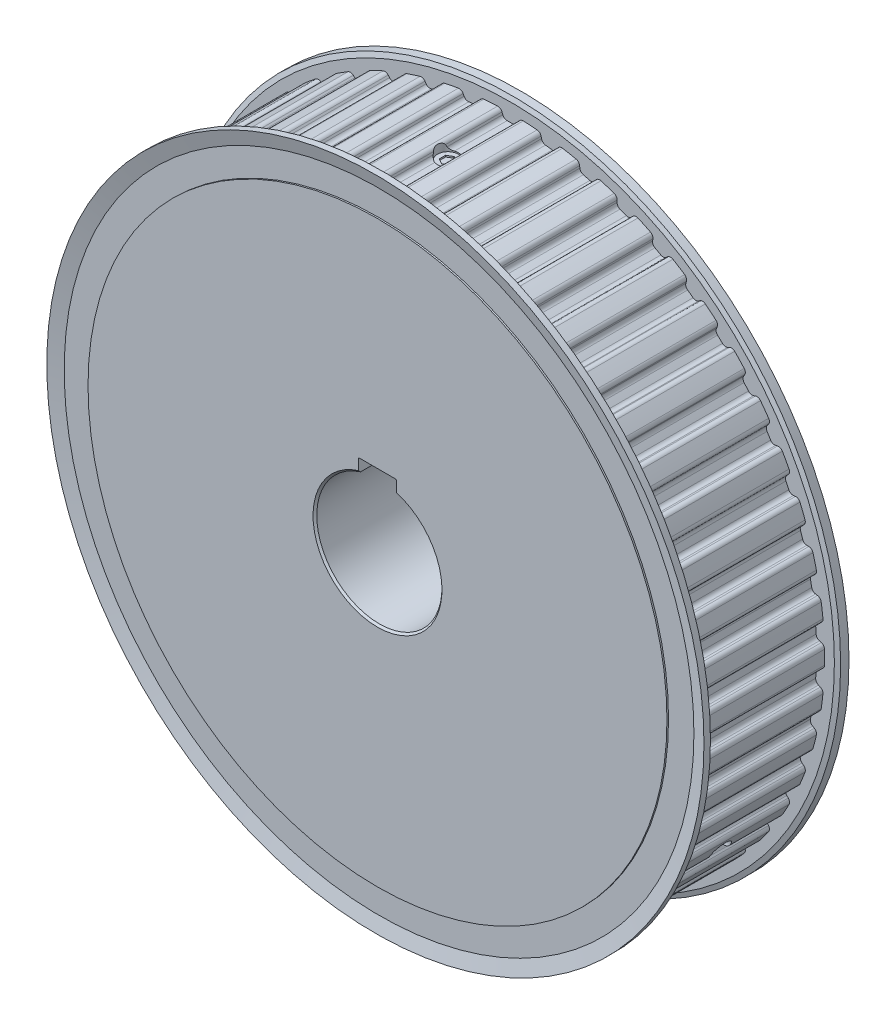
SolidWorks part; units mm, degrees
ref_plane "前视基准面" through (0, 0, 0) normal (0, 0, 1) x (1, 0, 0)
ref_plane "上视基准面" through (0, 0, 0) normal (0, 1, 0) x (1, 0, 0)
ref_plane "右视基准面" through (0, 0, 0) normal (1, 0, 0) x (0, 0, -1)
sketch "草图1" plane through (0, 0, 0) normal (1, 0, 0) x (0, 0, -1)
  line L0 (0, 0) -> (0, 92.5)
  line L1 (0, 92.5) -> (2.5, 92.5)
  line L2 (2.5, 92.5) -> (2.5, 102.38)
  line L3 (2.5, 102.38) -> (42.5, 102.38)
  line L4 (42.5, 102.38) -> (42.5, 92.5)
  line L5 (42.5, 92.5) -> (45, 92.5)
  line L6 (45, 92.5) -> (45, 0)
  line L7 (45, 0) -> (0, 0)
  line L8 (45, 0) -> (0, 0) construction
revolve "旋转1" add sketch "草图1" angle 360 about L8
sketch "草图2" plane through (0, 0, 0) normal (1, 0, 0) x (0, 0, -1)
  line L0 (0, 0) -> (0, 20.6)
  line L1 (0, 20.6) -> (0.6, 20)
  line L2 (0.6, 20) -> (44.4, 20)
  line L3 (44.4, 20) -> (45, 20.6)
  line L4 (45, 20.6) -> (45, 0)
  line L5 (45, 0) -> (0, 0)
  line L6 (45, 0) -> (0, 0) construction
revolve "切除-旋转1" cut sketch "草图2" angle 360 about L6
sketch "草图3" plane through (0, 0, 0) normal (1, 0, 0) x (0, 0, -1)
  line L0 (42.5, 103.5) -> (42.5, 92.5)
  line L1 (42.5, 92.5) -> (44.5, 92.5)
  line L2 (44.5, 92.5) -> (44.5, 105)
  line L3 (44.5, 105) -> (43, 105)
  line L4 (43, 105) -> (42.5, 103.5)
  line L5 (50, 0) -> (-50, 0) construction
revolve "旋转2" add sketch "草图3" angle 360 about L5
ref_plane "基准面1" through (0, 0, -22.5) normal (0, 0, 1) x (1, 0, 0)
sketch "草图4" plane through (0, 0, -22.5) normal (0, 0, 1) x (1, 0, 0)
  line L0 (-99.3369, -3.5434) -> (-98.7119, -3.7273)
  line L1 (-98.4007, -8.6739) -> (-98.9977, -8.9348)
  line L2 (-98.1095, -15.9657) -> (-97.4664, -16.0698)
  line L3 (-96.5376, -20.9384) -> (-97.0972, -21.272)
  line L4 (-95.3348, -28.1361) -> (-94.6838, -28.1589)
  line L5 (-93.1521, -32.8727) -> (-93.6655, -33.2738)
  line L6 (-91.0567, -39.8629) -> (-90.4079, -39.8039)
  line L7 (-88.2976, -44.2885) -> (-88.7566, -44.7508)
  line L8 (-85.3425, -50.961) -> (-84.7063, -50.8211)
  line L9 (-82.0505, -55.0059) -> (-82.448, -55.5221)
  line L10 (-78.2825, -61.2554) -> (-77.6687, -61.0369)
  line L11 (-74.5094, -64.8559) -> (-74.8391, -65.4178)
  line L12 (-69.9879, -70.5838) -> (-69.4064, -70.2901)
  line L13 (-65.7933, -73.683) -> (-66.0499, -74.2817)
  line L14 (-60.5895, -78.799) -> (-60.0494, -78.4347)
  line L15 (-56.0396, -81.348) -> (-56.2191, -81.9743)
  line L16 (-50.2356, -85.7715) -> (-49.7454, -85.3424)
  line L17 (-45.4021, -87.7302) -> (-45.5017, -88.374)
  line L18 (-39.0894, -91.3914) -> (-38.6569, -90.9042)
  line L19 (-34.0486, -92.7288) -> (-34.0667, -93.38)
  line L20 (-27.3268, -95.57) -> (-26.9588, -95.0324)
  line L21 (-22.1581, -96.265) -> (-22.0945, -96.9134)
  line L22 (-15.1333, -98.2413) -> (-14.8355, -97.6619)
  line L23 (-9.9181, -98.2831) -> (-9.7738, -98.9184)
  line L24 (-2.701, -99.3634) -> (-2.4782, -98.7512)
  line L25 (2.4782, -98.7512) -> (2.701, -99.3634)
  line L26 (9.7738, -98.9184) -> (9.9181, -98.2831)
  line L27 (14.8355, -97.6619) -> (15.1333, -98.2413)
  line L28 (22.0945, -96.9134) -> (22.1581, -96.265)
  line L29 (26.9588, -95.0324) -> (27.3268, -95.57)
  line L30 (34.0667, -93.38) -> (34.0486, -92.7288)
  line L31 (38.6569, -90.9042) -> (39.0894, -91.3914)
  line L32 (45.5017, -88.374) -> (45.4021, -87.7302)
  line L33 (49.7454, -85.3424) -> (50.2356, -85.7715)
  line L34 (56.2191, -81.9743) -> (56.0396, -81.348)
  line L35 (60.0494, -78.4347) -> (60.5895, -78.799)
  line L36 (66.0499, -74.2817) -> (65.7933, -73.683)
  line L37 (69.4064, -70.2901) -> (69.9879, -70.5838)
  line L38 (74.8391, -65.4178) -> (74.5094, -64.8559)
  line L39 (77.6687, -61.0369) -> (78.2825, -61.2554)
  line L40 (82.448, -55.5221) -> (82.0505, -55.0059)
  line L41 (84.7063, -50.8211) -> (85.3425, -50.961)
  line L42 (88.7566, -44.7508) -> (88.2976, -44.2885)
  line L43 (90.4079, -39.8039) -> (91.0567, -39.8629)
  line L44 (93.6655, -33.2738) -> (93.1521, -32.8727)
  line L45 (94.6838, -28.1589) -> (95.3348, -28.1361)
  line L46 (97.0972, -21.272) -> (96.5376, -20.9384)
  line L47 (97.4664, -16.0698) -> (98.1095, -15.9657)
  line L48 (98.9977, -8.9348) -> (98.4007, -8.6739)
  line L49 (98.7119, -3.7273) -> (99.3369, -3.5434)
  line L50 (99.3369, 3.5434) -> (98.7119, 3.7273)
  line L51 (98.4007, 8.6739) -> (98.9977, 8.9348)
  line L52 (98.1095, 15.9657) -> (97.4664, 16.0698)
  line L53 (96.5376, 20.9384) -> (97.0972, 21.272)
  line L54 (95.3348, 28.1361) -> (94.6838, 28.1589)
  line L55 (93.1521, 32.8727) -> (93.6655, 33.2738)
  line L56 (91.0567, 39.8629) -> (90.4079, 39.8039)
  line L57 (88.2976, 44.2885) -> (88.7566, 44.7508)
  line L58 (85.3425, 50.961) -> (84.7063, 50.8211)
  line L59 (82.0505, 55.0059) -> (82.448, 55.5221)
  line L60 (78.2825, 61.2554) -> (77.6687, 61.0369)
  line L61 (74.5094, 64.8559) -> (74.8391, 65.4178)
  line L62 (69.9879, 70.5838) -> (69.4064, 70.2901)
  line L63 (65.7933, 73.683) -> (66.0499, 74.2817)
  line L64 (60.5895, 78.799) -> (60.0494, 78.4347)
  line L65 (56.0396, 81.348) -> (56.2191, 81.9743)
  line L66 (50.2356, 85.7715) -> (49.7454, 85.3424)
  line L67 (45.4021, 87.7302) -> (45.5017, 88.374)
  line L68 (39.0894, 91.3914) -> (38.6569, 90.9042)
  line L69 (34.0486, 92.7288) -> (34.0667, 93.38)
  line L70 (27.3268, 95.57) -> (26.9588, 95.0324)
  line L71 (22.1581, 96.265) -> (22.0945, 96.9134)
  line L72 (15.1333, 98.2413) -> (14.8355, 97.6619)
  line L73 (9.9181, 98.2831) -> (9.7738, 98.9184)
  line L74 (2.701, 99.3634) -> (2.4782, 98.7512)
  line L75 (-2.4782, 98.7512) -> (-2.701, 99.3634)
  line L76 (-9.7738, 98.9184) -> (-9.9181, 98.2831)
  line L77 (-14.8355, 97.6619) -> (-15.1333, 98.2413)
  line L78 (-22.0945, 96.9134) -> (-22.1581, 96.265)
  line L79 (-26.9588, 95.0324) -> (-27.3268, 95.57)
  line L80 (-34.0667, 93.38) -> (-34.0486, 92.7288)
  line L81 (-38.6569, 90.9042) -> (-39.0894, 91.3914)
  line L82 (-45.5017, 88.374) -> (-45.4021, 87.7302)
  line L83 (-49.7454, 85.3424) -> (-50.2356, 85.7715)
  line L84 (-56.2191, 81.9743) -> (-56.0396, 81.348)
  line L85 (-60.0494, 78.4347) -> (-60.5895, 78.799)
  line L86 (-66.0499, 74.2817) -> (-65.7933, 73.683)
  line L87 (-69.4064, 70.2901) -> (-69.9879, 70.5838)
  line L88 (-74.8391, 65.4178) -> (-74.5094, 64.8559)
  line L89 (-77.6687, 61.0369) -> (-78.2825, 61.2554)
  line L90 (-82.448, 55.5221) -> (-82.0505, 55.0059)
  line L91 (-84.7063, 50.8211) -> (-85.3425, 50.961)
  line L92 (-88.7566, 44.7508) -> (-88.2976, 44.2885)
  line L93 (-90.4079, 39.8039) -> (-91.0567, 39.8629)
  line L94 (-93.6655, 33.2738) -> (-93.1521, 32.8727)
  line L95 (-94.6838, 28.1589) -> (-95.3348, 28.1361)
  line L96 (-97.0972, 21.272) -> (-96.5376, 20.9384)
  line L97 (-97.4664, 16.0698) -> (-98.1095, 15.9657)
  line L98 (-98.9977, 8.9348) -> (-98.4007, 8.6739)
  line L99 (-98.7119, 3.7273) -> (-99.3369, 3.5434)
  circle A0 centre (0, 0) radius 200.76
  arc A1 (-100.3556, 2.2125) -> (-100.3556, -2.2125) centre (0, 0) ccw
  arc A2 (-100.3556, -2.2125) -> (-99.3369, -3.5434) centre (-98.936, -2.1812) ccw
  arc A3 (-98.7119, -3.7273) -> (-97.6589, -5.0614) centre (-99.127, -5.1375) cw
  arc A4 (-97.6589, -5.0614) -> (-97.5232, -7.2184) centre (0, 0) ccw
  arc A5 (-97.5232, -7.2184) -> (-98.4007, -8.6739) centre (-98.9892, -7.3269) cw
  arc A6 (-98.9977, -8.9348) -> (-99.8416, -10.3829) centre (-98.4292, -10.236) ccw
  arc A7 (-99.8416, -10.3829) -> (-99.287, -14.7729) centre (0, 0) ccw
  arc A8 (-99.287, -14.7729) -> (-98.1095, -15.9657) centre (-97.8824, -14.5639) ccw
  arc A9 (-97.4664, -16.0698) -> (-96.2545, -17.2614) centre (-97.7014, -17.5209) cw
  arc A10 (-96.2545, -17.2614) -> (-95.8495, -19.3844) centre (0, 0) ccw
  arc A11 (-95.8495, -19.3844) -> (-96.5376, -20.9384) centre (-97.2903, -19.6758) cw
  arc A12 (-97.0972, -21.272) -> (-97.753, -22.8145) centre (-96.3701, -22.4917) ccw
  arc A13 (-97.753, -22.8145) -> (-96.6525, -27.1004) centre (0, 0) ccw
  arc A14 (-96.6525, -27.1004) -> (-95.3348, -28.1361) centre (-95.2853, -26.717) ccw
  arc A15 (-94.6838, -28.1589) -> (-93.3321, -29.1892) centre (-94.7351, -29.628) cw
  arc A16 (-93.3321, -29.1892) -> (-92.6642, -31.2446) centre (0, 0) ccw
  arc A17 (-92.6642, -31.2446) -> (-93.1521, -32.8727) centre (-94.0572, -31.7143) cw
  arc A18 (-93.6655, -33.2738) -> (-94.1228, -34.8863) centre (-92.7913, -34.3928) ccw
  arc A19 (-94.1228, -34.8863) -> (-92.4938, -39.0005) centre (0, 0) ccw
  arc A20 (-92.4938, -39.0005) -> (-91.0567, -39.8629) centre (-91.1854, -38.4487) ccw
  arc A21 (-90.4079, -39.8039) -> (-88.9377, -40.6566) centre (-90.2747, -41.2678) cw
  arc A22 (-88.9377, -40.6566) -> (-88.0175, -42.6122) centre (0, 0) ccw
  arc A23 (-88.0175, -42.6122) -> (-88.2976, -44.2885) centre (-89.3406, -43.2527) cw
  arc A24 (-88.7566, -44.7508) -> (-89.0082, -46.4079) centre (-87.749, -45.7514) ccw
  arc A25 (-89.0082, -46.4079) -> (-86.8764, -50.2855) centre (0, 0) ccw
  arc A26 (-86.8764, -50.2855) -> (-85.3425, -50.961) centre (-85.6475, -49.5741) ccw
  arc A27 (-84.7063, -50.8211) -> (-83.1408, -51.4829) centre (-84.3906, -52.2568) cw
  arc A28 (-83.1408, -51.4829) -> (-81.9828, -53.3077) centre (0, 0) ccw
  arc A29 (-81.9828, -53.3077) -> (-82.0505, -55.0059) centre (-83.2151, -54.109) cw
  arc A30 (-82.448, -55.5221) -> (-82.4898, -57.1976) centre (-81.3229, -56.3885) ccw
  arc A31 (-82.4898, -57.1976) -> (-79.8889, -60.7775) centre (0, 0) ccw
  arc A32 (-79.8889, -60.7775) -> (-78.2825, -61.2554) centre (-78.7588, -59.9177) ccw
  arc A33 (-77.6687, -61.0369) -> (-76.0327, -61.4973) centre (-77.1756, -62.4217) cw
  arc A34 (-76.0327, -61.4973) -> (-74.6551, -63.1625) centre (0, 0) ccw
  arc A35 (-74.6551, -63.1625) -> (-74.5094, -64.8559) centre (-75.7773, -64.112) cw
  arc A36 (-74.8391, -65.4178) -> (-74.6706, -67.0853) centre (-73.6143, -66.1363) ccw
  arc A37 (-74.6706, -67.0853) -> (-71.6416, -70.311) centre (0, 0) ccw
  arc A38 (-71.6416, -70.311) -> (-69.9879, -70.5838) centre (-70.6281, -69.3163) ccw
  arc A39 (-69.4064, -70.2901) -> (-67.7255, -70.5418) centre (-68.7436, -71.6022) cw
  arc A40 (-67.7255, -70.5418) -> (-66.15, -72.0212) centre (0, 0) ccw
  arc A41 (-66.15, -72.0212) -> (-65.7933, -73.683) centre (-67.1444, -73.1039) cw
  arc A42 (-66.0499, -74.2817) -> (-65.6738, -75.9151) centre (-64.7448, -74.8411) ccw
  arc A43 (-65.6738, -75.9151) -> (-62.2643, -78.7356) centre (0, 0) ccw
  arc A44 (-62.2643, -78.7356) -> (-60.5895, -78.799) centre (-61.3835, -77.6218) ccw
  arc A45 (-60.0494, -78.4347) -> (-58.3502, -78.4738) centre (-59.2274, -79.6534) cw
  arc A46 (-58.3502, -78.4738) -> (-56.6018, -79.7441) centre (0, 0) ccw
  arc A47 (-56.6018, -79.7441) -> (-56.0396, -81.348) centre (-57.4526, -80.9428) cw
  arc A48 (-56.2191, -81.9743) -> (-55.6413, -83.5476) centre (-54.8542, -82.3657) ccw
  arc A49 (-55.6413, -83.5476) -> (-51.9052, -85.9185) centre (0, 0) ccw
  arc A50 (-51.9052, -85.9185) -> (-50.2356, -85.7715) centre (-51.1709, -84.7031) ccw
  arc A51 (-49.7454, -85.3424) -> (-48.0548, -85.1682) centre (-48.7771, -86.4485) cw
  arc A52 (-48.0548, -85.1682) -> (-46.1609, -86.2094) centre (0, 0) ccw
  arc A53 (-46.1609, -86.2094) -> (-45.4021, -87.7302) centre (-46.8548, -87.5053) cw
  arc A54 (-45.5017, -88.374) -> (-44.7312, -89.8625) centre (-44.0985, -88.5912) ccw
  arc A55 (-44.7312, -89.8625) -> (-40.7275, -91.7465) centre (0, 0) ccw
  arc A56 (-40.7275, -91.7465) -> (-39.0894, -91.3914) centre (-40.1513, -90.4486) ccw
  arc A57 (-38.6569, -90.9042) -> (-37.0014, -90.5195) centre (-37.5576, -91.8802) cw
  arc A58 (-37.0014, -90.5195) -> (-34.992, -91.3151) centre (0, 0) ccw
  arc A59 (-34.992, -91.3151) -> (-34.0486, -92.7288) centre (-35.518, -92.6878) cw
  arc A60 (-34.0667, -93.38) -> (-33.1158, -94.7602) centre (-32.6473, -93.4197) ccw
  arc A61 (-33.1158, -94.7602) -> (-28.9074, -96.1275) centre (0, 0) ccw
  arc A62 (-28.9074, -96.1275) -> (-27.3268, -95.57) centre (-28.4985, -94.7677) ccw
  arc A63 (-26.9588, -95.0324) -> (-25.3646, -94.4432) centre (-25.7458, -95.8629) cw
  arc A64 (-25.3646, -94.4432) -> (-23.2712, -94.9807) centre (0, 0) ccw
  arc A65 (-23.2712, -94.9807) -> (-22.1581, -96.265) centre (-23.6211, -96.4085) cw
  arc A66 (-22.0945, -96.9134) -> (-20.978, -98.1635) centre (-20.6813, -96.7748) ccw
  arc A67 (-20.978, -98.1635) -> (-16.6315, -98.9926) centre (0, 0) ccw
  arc A68 (-16.6315, -98.9926) -> (-15.1333, -98.2413) centre (-16.3962, -97.5922) ccw
  arc A69 (-14.8355, -97.6619) -> (-13.3277, -96.8775) centre (-13.528, -98.3338) cw
  arc A70 (-13.3277, -96.8775) -> (-11.1835, -97.1484) centre (0, 0) ccw
  arc A71 (-11.1835, -97.1484) -> (-9.9181, -98.2831) centre (-11.3516, -98.6088) cw
  arc A72 (-9.7738, -98.9184) -> (-8.5095, -100.0187) centre (-8.3891, -98.6038) ccw
  arc A73 (-8.5095, -100.0187) -> (-4.0933, -100.2965) centre (0, 0) ccw
  arc A74 (-4.0933, -100.2965) -> (-2.701, -99.3634) centre (-4.0354, -98.8777) ccw
  arc A75 (-2.4782, -98.7512) -> (-1.0806, -97.784) centre (-1.0969, -99.2539) cw
  arc A76 (-1.0806, -97.784) -> (1.0806, -97.784) centre (0, 0) ccw
  arc A77 (1.0806, -97.784) -> (2.4782, -98.7512) centre (1.0969, -99.2539) cw
  arc A78 (2.701, -99.3634) -> (4.0933, -100.2965) centre (4.0354, -98.8777) ccw
  arc A79 (4.0933, -100.2965) -> (8.5095, -100.0187) centre (0, 0) ccw
  arc A80 (8.5095, -100.0187) -> (9.7738, -98.9184) centre (8.3891, -98.6038) ccw
  arc A81 (9.9181, -98.2831) -> (11.1835, -97.1484) centre (11.3516, -98.6088) cw
  arc A82 (11.1835, -97.1484) -> (13.3277, -96.8775) centre (0, 0) ccw
  arc A83 (13.3277, -96.8775) -> (14.8355, -97.6619) centre (13.528, -98.3338) cw
  arc A84 (15.1333, -98.2413) -> (16.6315, -98.9926) centre (16.3962, -97.5922) ccw
  arc A85 (16.6315, -98.9926) -> (20.978, -98.1635) centre (0, 0) ccw
  arc A86 (20.978, -98.1635) -> (22.0945, -96.9134) centre (20.6813, -96.7748) ccw
  arc A87 (22.1581, -96.265) -> (23.2712, -94.9807) centre (23.6211, -96.4085) cw
  arc A88 (23.2712, -94.9807) -> (25.3646, -94.4432) centre (0, 0) ccw
  arc A89 (25.3646, -94.4432) -> (26.9588, -95.0324) centre (25.7458, -95.8629) cw
  arc A90 (27.3268, -95.57) -> (28.9074, -96.1275) centre (28.4985, -94.7677) ccw
  arc A91 (28.9074, -96.1275) -> (33.1158, -94.7602) centre (0, 0) ccw
  arc A92 (33.1158, -94.7602) -> (34.0667, -93.38) centre (32.6473, -93.4197) ccw
  arc A93 (34.0486, -92.7288) -> (34.992, -91.3151) centre (35.518, -92.6878) cw
  arc A94 (34.992, -91.3151) -> (37.0014, -90.5195) centre (0, 0) ccw
  arc A95 (37.0014, -90.5195) -> (38.6569, -90.9042) centre (37.5576, -91.8802) cw
  arc A96 (39.0894, -91.3914) -> (40.7275, -91.7465) centre (40.1513, -90.4486) ccw
  arc A97 (40.7275, -91.7465) -> (44.7312, -89.8625) centre (0, 0) ccw
  arc A98 (44.7312, -89.8625) -> (45.5017, -88.374) centre (44.0985, -88.5912) ccw
  arc A99 (45.4021, -87.7302) -> (46.1609, -86.2094) centre (46.8548, -87.5053) cw
  arc A100 (46.1609, -86.2094) -> (48.0548, -85.1682) centre (0, 0) ccw
  arc A101 (48.0548, -85.1682) -> (49.7454, -85.3424) centre (48.7771, -86.4485) cw
  arc A102 (50.2356, -85.7715) -> (51.9052, -85.9185) centre (51.1709, -84.7031) ccw
  arc A103 (51.9052, -85.9185) -> (55.6413, -83.5476) centre (0, 0) ccw
  arc A104 (55.6413, -83.5476) -> (56.2191, -81.9743) centre (54.8542, -82.3657) ccw
  arc A105 (56.0396, -81.348) -> (56.6018, -79.7441) centre (57.4526, -80.9428) cw
  arc A106 (56.6018, -79.7441) -> (58.3502, -78.4738) centre (0, 0) ccw
  arc A107 (58.3502, -78.4738) -> (60.0494, -78.4347) centre (59.2274, -79.6534) cw
  arc A108 (60.5895, -78.799) -> (62.2643, -78.7356) centre (61.3835, -77.6218) ccw
  arc A109 (62.2643, -78.7356) -> (65.6738, -75.9151) centre (0, 0) ccw
  arc A110 (65.6738, -75.9151) -> (66.0499, -74.2817) centre (64.7448, -74.8411) ccw
  arc A111 (65.7933, -73.683) -> (66.15, -72.0212) centre (67.1444, -73.1039) cw
  arc A112 (66.15, -72.0212) -> (67.7255, -70.5418) centre (0, 0) ccw
  arc A113 (67.7255, -70.5418) -> (69.4064, -70.2901) centre (68.7436, -71.6022) cw
  arc A114 (69.9879, -70.5838) -> (71.6416, -70.311) centre (70.6281, -69.3163) ccw
  arc A115 (71.6416, -70.311) -> (74.6706, -67.0853) centre (0, 0) ccw
  arc A116 (74.6706, -67.0853) -> (74.8391, -65.4178) centre (73.6143, -66.1363) ccw
  arc A117 (74.5094, -64.8559) -> (74.6551, -63.1625) centre (75.7773, -64.112) cw
  arc A118 (74.6551, -63.1625) -> (76.0327, -61.4973) centre (0, 0) ccw
  arc A119 (76.0327, -61.4973) -> (77.6687, -61.0369) centre (77.1756, -62.4217) cw
  arc A120 (78.2825, -61.2554) -> (79.8889, -60.7775) centre (78.7588, -59.9177) ccw
  arc A121 (79.8889, -60.7775) -> (82.4898, -57.1976) centre (0, 0) ccw
  arc A122 (82.4898, -57.1976) -> (82.448, -55.5221) centre (81.3229, -56.3885) ccw
  arc A123 (82.0505, -55.0059) -> (81.9828, -53.3077) centre (83.2151, -54.109) cw
  arc A124 (81.9828, -53.3077) -> (83.1408, -51.4829) centre (0, 0) ccw
  arc A125 (83.1408, -51.4829) -> (84.7063, -50.8211) centre (84.3906, -52.2568) cw
  arc A126 (85.3425, -50.961) -> (86.8764, -50.2855) centre (85.6475, -49.5741) ccw
  arc A127 (86.8764, -50.2855) -> (89.0082, -46.4079) centre (0, 0) ccw
  arc A128 (89.0082, -46.4079) -> (88.7566, -44.7508) centre (87.749, -45.7514) ccw
  arc A129 (88.2976, -44.2885) -> (88.0175, -42.6122) centre (89.3406, -43.2527) cw
  arc A130 (88.0175, -42.6122) -> (88.9377, -40.6566) centre (0, 0) ccw
  arc A131 (88.9377, -40.6566) -> (90.4079, -39.8039) centre (90.2747, -41.2678) cw
  arc A132 (91.0567, -39.8629) -> (92.4938, -39.0005) centre (91.1854, -38.4487) ccw
  arc A133 (92.4938, -39.0005) -> (94.1228, -34.8863) centre (0, 0) ccw
  arc A134 (94.1228, -34.8863) -> (93.6655, -33.2738) centre (92.7913, -34.3928) ccw
  arc A135 (93.1521, -32.8727) -> (92.6642, -31.2446) centre (94.0572, -31.7143) cw
  arc A136 (92.6642, -31.2446) -> (93.3321, -29.1892) centre (0, 0) ccw
  arc A137 (93.3321, -29.1892) -> (94.6838, -28.1589) centre (94.7351, -29.628) cw
  arc A138 (95.3348, -28.1361) -> (96.6525, -27.1004) centre (95.2853, -26.717) ccw
  arc A139 (96.6525, -27.1004) -> (97.753, -22.8145) centre (0, 0) ccw
  arc A140 (97.753, -22.8145) -> (97.0972, -21.272) centre (96.3701, -22.4917) ccw
  arc A141 (96.5376, -20.9384) -> (95.8495, -19.3844) centre (97.2903, -19.6758) cw
  arc A142 (95.8495, -19.3844) -> (96.2545, -17.2614) centre (0, 0) ccw
  arc A143 (96.2545, -17.2614) -> (97.4664, -16.0698) centre (97.7014, -17.5209) cw
  arc A144 (98.1095, -15.9657) -> (99.287, -14.7729) centre (97.8824, -14.5639) ccw
  arc A145 (99.287, -14.7729) -> (99.8416, -10.3829) centre (0, 0) ccw
  arc A146 (99.8416, -10.3829) -> (98.9977, -8.9348) centre (98.4292, -10.236) ccw
  arc A147 (98.4007, -8.6739) -> (97.5232, -7.2184) centre (98.9892, -7.3269) cw
  arc A148 (97.5232, -7.2184) -> (97.6589, -5.0614) centre (0, 0) ccw
  arc A149 (97.6589, -5.0614) -> (98.7119, -3.7273) centre (99.127, -5.1375) cw
  arc A150 (99.3369, -3.5434) -> (100.3556, -2.2125) centre (98.936, -2.1812) ccw
  arc A151 (100.3556, -2.2125) -> (100.3556, 2.2125) centre (0, 0) ccw
  arc A152 (100.3556, 2.2125) -> (99.3369, 3.5434) centre (98.936, 2.1812) ccw
  arc A153 (98.7119, 3.7273) -> (97.6589, 5.0614) centre (99.127, 5.1375) cw
  arc A154 (97.6589, 5.0614) -> (97.5232, 7.2184) centre (0, 0) ccw
  arc A155 (97.5232, 7.2184) -> (98.4007, 8.6739) centre (98.9892, 7.3269) cw
  arc A156 (98.9977, 8.9348) -> (99.8416, 10.3829) centre (98.4292, 10.236) ccw
  arc A157 (99.8416, 10.3829) -> (99.287, 14.7729) centre (0, 0) ccw
  arc A158 (99.287, 14.7729) -> (98.1095, 15.9657) centre (97.8824, 14.5639) ccw
  arc A159 (97.4664, 16.0698) -> (96.2545, 17.2614) centre (97.7014, 17.5209) cw
  arc A160 (96.2545, 17.2614) -> (95.8495, 19.3844) centre (0, 0) ccw
  arc A161 (95.8495, 19.3844) -> (96.5376, 20.9384) centre (97.2903, 19.6758) cw
  arc A162 (97.0972, 21.272) -> (97.753, 22.8145) centre (96.3701, 22.4917) ccw
  arc A163 (97.753, 22.8145) -> (96.6525, 27.1004) centre (0, 0) ccw
  arc A164 (96.6525, 27.1004) -> (95.3348, 28.1361) centre (95.2853, 26.717) ccw
  arc A165 (94.6838, 28.1589) -> (93.3321, 29.1892) centre (94.7351, 29.628) cw
  arc A166 (93.3321, 29.1892) -> (92.6642, 31.2446) centre (0, 0) ccw
  arc A167 (92.6642, 31.2446) -> (93.1521, 32.8727) centre (94.0572, 31.7143) cw
  arc A168 (93.6655, 33.2738) -> (94.1228, 34.8863) centre (92.7913, 34.3928) ccw
  arc A169 (94.1228, 34.8863) -> (92.4938, 39.0005) centre (0, 0) ccw
  arc A170 (92.4938, 39.0005) -> (91.0567, 39.8629) centre (91.1854, 38.4487) ccw
  arc A171 (90.4079, 39.8039) -> (88.9377, 40.6566) centre (90.2747, 41.2678) cw
  arc A172 (88.9377, 40.6566) -> (88.0175, 42.6122) centre (0, 0) ccw
  arc A173 (88.0175, 42.6122) -> (88.2976, 44.2885) centre (89.3406, 43.2527) cw
  arc A174 (88.7566, 44.7508) -> (89.0082, 46.4079) centre (87.749, 45.7514) ccw
  arc A175 (89.0082, 46.4079) -> (86.8764, 50.2855) centre (0, 0) ccw
  arc A176 (86.8764, 50.2855) -> (85.3425, 50.961) centre (85.6475, 49.5741) ccw
  arc A177 (84.7063, 50.8211) -> (83.1408, 51.4829) centre (84.3906, 52.2568) cw
  arc A178 (83.1408, 51.4829) -> (81.9828, 53.3077) centre (0, 0) ccw
  arc A179 (81.9828, 53.3077) -> (82.0505, 55.0059) centre (83.2151, 54.109) cw
  arc A180 (82.448, 55.5221) -> (82.4898, 57.1976) centre (81.3229, 56.3885) ccw
  arc A181 (82.4898, 57.1976) -> (79.8889, 60.7775) centre (0, 0) ccw
  arc A182 (79.8889, 60.7775) -> (78.2825, 61.2554) centre (78.7588, 59.9177) ccw
  arc A183 (77.6687, 61.0369) -> (76.0327, 61.4973) centre (77.1756, 62.4217) cw
  arc A184 (76.0327, 61.4973) -> (74.6551, 63.1625) centre (0, 0) ccw
  arc A185 (74.6551, 63.1625) -> (74.5094, 64.8559) centre (75.7773, 64.112) cw
  arc A186 (74.8391, 65.4178) -> (74.6706, 67.0853) centre (73.6143, 66.1363) ccw
  arc A187 (74.6706, 67.0853) -> (71.6416, 70.311) centre (0, 0) ccw
  arc A188 (71.6416, 70.311) -> (69.9879, 70.5838) centre (70.6281, 69.3163) ccw
  arc A189 (69.4064, 70.2901) -> (67.7255, 70.5418) centre (68.7436, 71.6022) cw
  arc A190 (67.7255, 70.5418) -> (66.15, 72.0212) centre (0, 0) ccw
  arc A191 (66.15, 72.0212) -> (65.7933, 73.683) centre (67.1444, 73.1039) cw
  arc A192 (66.0499, 74.2817) -> (65.6738, 75.9151) centre (64.7448, 74.8411) ccw
  arc A193 (65.6738, 75.9151) -> (62.2643, 78.7356) centre (0, 0) ccw
  arc A194 (62.2643, 78.7356) -> (60.5895, 78.799) centre (61.3835, 77.6218) ccw
  arc A195 (60.0494, 78.4347) -> (58.3502, 78.4738) centre (59.2274, 79.6534) cw
  arc A196 (58.3502, 78.4738) -> (56.6018, 79.7441) centre (0, 0) ccw
  arc A197 (56.6018, 79.7441) -> (56.0396, 81.348) centre (57.4526, 80.9428) cw
  arc A198 (56.2191, 81.9743) -> (55.6413, 83.5476) centre (54.8542, 82.3657) ccw
  arc A199 (55.6413, 83.5476) -> (51.9052, 85.9185) centre (0, 0) ccw
  arc A200 (51.9052, 85.9185) -> (50.2356, 85.7715) centre (51.1709, 84.7031) ccw
  arc A201 (49.7454, 85.3424) -> (48.0548, 85.1682) centre (48.7771, 86.4485) cw
  arc A202 (48.0548, 85.1682) -> (46.1609, 86.2094) centre (0, 0) ccw
  arc A203 (46.1609, 86.2094) -> (45.4021, 87.7302) centre (46.8548, 87.5053) cw
  arc A204 (45.5017, 88.374) -> (44.7312, 89.8625) centre (44.0985, 88.5912) ccw
  arc A205 (44.7312, 89.8625) -> (40.7275, 91.7465) centre (0, 0) ccw
  arc A206 (40.7275, 91.7465) -> (39.0894, 91.3914) centre (40.1513, 90.4486) ccw
  arc A207 (38.6569, 90.9042) -> (37.0014, 90.5195) centre (37.5576, 91.8802) cw
  arc A208 (37.0014, 90.5195) -> (34.992, 91.3151) centre (0, 0) ccw
  arc A209 (34.992, 91.3151) -> (34.0486, 92.7288) centre (35.518, 92.6878) cw
  arc A210 (34.0667, 93.38) -> (33.1158, 94.7602) centre (32.6473, 93.4197) ccw
  arc A211 (33.1158, 94.7602) -> (28.9074, 96.1275) centre (0, 0) ccw
  arc A212 (28.9074, 96.1275) -> (27.3268, 95.57) centre (28.4985, 94.7677) ccw
  arc A213 (26.9588, 95.0324) -> (25.3646, 94.4432) centre (25.7458, 95.8629) cw
  arc A214 (25.3646, 94.4432) -> (23.2712, 94.9807) centre (0, 0) ccw
  arc A215 (23.2712, 94.9807) -> (22.1581, 96.265) centre (23.6211, 96.4085) cw
  arc A216 (22.0945, 96.9134) -> (20.978, 98.1635) centre (20.6813, 96.7748) ccw
  arc A217 (20.978, 98.1635) -> (16.6315, 98.9926) centre (0, 0) ccw
  arc A218 (16.6315, 98.9926) -> (15.1333, 98.2413) centre (16.3962, 97.5922) ccw
  arc A219 (14.8355, 97.6619) -> (13.3277, 96.8775) centre (13.528, 98.3338) cw
  arc A220 (13.3277, 96.8775) -> (11.1835, 97.1484) centre (0, 0) ccw
  arc A221 (11.1835, 97.1484) -> (9.9181, 98.2831) centre (11.3516, 98.6088) cw
  arc A222 (9.7738, 98.9184) -> (8.5095, 100.0187) centre (8.3891, 98.6038) ccw
  arc A223 (8.5095, 100.0187) -> (4.0933, 100.2965) centre (0, 0) ccw
  arc A224 (4.0933, 100.2965) -> (2.701, 99.3634) centre (4.0354, 98.8777) ccw
  arc A225 (2.4782, 98.7512) -> (1.0806, 97.784) centre (1.0969, 99.2539) cw
  arc A226 (1.0806, 97.784) -> (-1.0806, 97.784) centre (0, 0) ccw
  arc A227 (-1.0806, 97.784) -> (-2.4782, 98.7512) centre (-1.0969, 99.2539) cw
  arc A228 (-2.701, 99.3634) -> (-4.0933, 100.2965) centre (-4.0354, 98.8777) ccw
  arc A229 (-4.0933, 100.2965) -> (-8.5095, 100.0187) centre (0, 0) ccw
  arc A230 (-8.5095, 100.0187) -> (-9.7738, 98.9184) centre (-8.3891, 98.6038) ccw
  arc A231 (-9.9181, 98.2831) -> (-11.1835, 97.1484) centre (-11.3516, 98.6088) cw
  arc A232 (-11.1835, 97.1484) -> (-13.3277, 96.8775) centre (0, 0) ccw
  arc A233 (-13.3277, 96.8775) -> (-14.8355, 97.6619) centre (-13.528, 98.3338) cw
  arc A234 (-15.1333, 98.2413) -> (-16.6315, 98.9926) centre (-16.3962, 97.5922) ccw
  arc A235 (-16.6315, 98.9926) -> (-20.978, 98.1635) centre (0, 0) ccw
  arc A236 (-20.978, 98.1635) -> (-22.0945, 96.9134) centre (-20.6813, 96.7748) ccw
  arc A237 (-22.1581, 96.265) -> (-23.2712, 94.9807) centre (-23.6211, 96.4085) cw
  arc A238 (-23.2712, 94.9807) -> (-25.3646, 94.4432) centre (0, 0) ccw
  arc A239 (-25.3646, 94.4432) -> (-26.9588, 95.0324) centre (-25.7458, 95.8629) cw
  arc A240 (-27.3268, 95.57) -> (-28.9074, 96.1275) centre (-28.4985, 94.7677) ccw
  arc A241 (-28.9074, 96.1275) -> (-33.1158, 94.7602) centre (0, 0) ccw
  arc A242 (-33.1158, 94.7602) -> (-34.0667, 93.38) centre (-32.6473, 93.4197) ccw
  arc A243 (-34.0486, 92.7288) -> (-34.992, 91.3151) centre (-35.518, 92.6878) cw
  arc A244 (-34.992, 91.3151) -> (-37.0014, 90.5195) centre (0, 0) ccw
  arc A245 (-37.0014, 90.5195) -> (-38.6569, 90.9042) centre (-37.5576, 91.8802) cw
  arc A246 (-39.0894, 91.3914) -> (-40.7275, 91.7465) centre (-40.1513, 90.4486) ccw
  arc A247 (-40.7275, 91.7465) -> (-44.7312, 89.8625) centre (0, 0) ccw
  arc A248 (-44.7312, 89.8625) -> (-45.5017, 88.374) centre (-44.0985, 88.5912) ccw
  arc A249 (-45.4021, 87.7302) -> (-46.1609, 86.2094) centre (-46.8548, 87.5053) cw
  arc A250 (-46.1609, 86.2094) -> (-48.0548, 85.1682) centre (0, 0) ccw
  arc A251 (-48.0548, 85.1682) -> (-49.7454, 85.3424) centre (-48.7771, 86.4485) cw
  arc A252 (-50.2356, 85.7715) -> (-51.9052, 85.9185) centre (-51.1709, 84.7031) ccw
  arc A253 (-51.9052, 85.9185) -> (-55.6413, 83.5476) centre (0, 0) ccw
  arc A254 (-55.6413, 83.5476) -> (-56.2191, 81.9743) centre (-54.8542, 82.3657) ccw
  arc A255 (-56.0396, 81.348) -> (-56.6018, 79.7441) centre (-57.4526, 80.9428) cw
  arc A256 (-56.6018, 79.7441) -> (-58.3502, 78.4738) centre (0, 0) ccw
  arc A257 (-58.3502, 78.4738) -> (-60.0494, 78.4347) centre (-59.2274, 79.6534) cw
  arc A258 (-60.5895, 78.799) -> (-62.2643, 78.7356) centre (-61.3835, 77.6218) ccw
  arc A259 (-62.2643, 78.7356) -> (-65.6738, 75.9151) centre (0, 0) ccw
  arc A260 (-65.6738, 75.9151) -> (-66.0499, 74.2817) centre (-64.7448, 74.8411) ccw
  arc A261 (-65.7933, 73.683) -> (-66.15, 72.0212) centre (-67.1444, 73.1039) cw
  arc A262 (-66.15, 72.0212) -> (-67.7255, 70.5418) centre (0, 0) ccw
  arc A263 (-67.7255, 70.5418) -> (-69.4064, 70.2901) centre (-68.7436, 71.6022) cw
  arc A264 (-69.9879, 70.5838) -> (-71.6416, 70.311) centre (-70.6281, 69.3163) ccw
  arc A265 (-71.6416, 70.311) -> (-74.6706, 67.0853) centre (0, 0) ccw
  arc A266 (-74.6706, 67.0853) -> (-74.8391, 65.4178) centre (-73.6143, 66.1363) ccw
  arc A267 (-74.5094, 64.8559) -> (-74.6551, 63.1625) centre (-75.7773, 64.112) cw
  arc A268 (-74.6551, 63.1625) -> (-76.0327, 61.4973) centre (0, 0) ccw
  arc A269 (-76.0327, 61.4973) -> (-77.6687, 61.0369) centre (-77.1756, 62.4217) cw
  arc A270 (-78.2825, 61.2554) -> (-79.8889, 60.7775) centre (-78.7588, 59.9177) ccw
  arc A271 (-79.8889, 60.7775) -> (-82.4898, 57.1976) centre (0, 0) ccw
  arc A272 (-82.4898, 57.1976) -> (-82.448, 55.5221) centre (-81.3229, 56.3885) ccw
  arc A273 (-82.0505, 55.0059) -> (-81.9828, 53.3077) centre (-83.2151, 54.109) cw
  arc A274 (-81.9828, 53.3077) -> (-83.1408, 51.4829) centre (0, 0) ccw
  arc A275 (-83.1408, 51.4829) -> (-84.7063, 50.8211) centre (-84.3906, 52.2568) cw
  arc A276 (-85.3425, 50.961) -> (-86.8764, 50.2855) centre (-85.6475, 49.5741) ccw
  arc A277 (-86.8764, 50.2855) -> (-89.0082, 46.4079) centre (0, 0) ccw
  arc A278 (-89.0082, 46.4079) -> (-88.7566, 44.7508) centre (-87.749, 45.7514) ccw
  arc A279 (-88.2976, 44.2885) -> (-88.0175, 42.6122) centre (-89.3406, 43.2527) cw
  arc A280 (-88.0175, 42.6122) -> (-88.9377, 40.6566) centre (0, 0) ccw
  arc A281 (-88.9377, 40.6566) -> (-90.4079, 39.8039) centre (-90.2747, 41.2678) cw
  arc A282 (-91.0567, 39.8629) -> (-92.4938, 39.0005) centre (-91.1854, 38.4487) ccw
  arc A283 (-92.4938, 39.0005) -> (-94.1228, 34.8863) centre (0, 0) ccw
  arc A284 (-94.1228, 34.8863) -> (-93.6655, 33.2738) centre (-92.7913, 34.3928) ccw
  arc A285 (-93.1521, 32.8727) -> (-92.6642, 31.2446) centre (-94.0572, 31.7143) cw
  arc A286 (-92.6642, 31.2446) -> (-93.3321, 29.1892) centre (0, 0) ccw
  arc A287 (-93.3321, 29.1892) -> (-94.6838, 28.1589) centre (-94.7351, 29.628) cw
  arc A288 (-95.3348, 28.1361) -> (-96.6525, 27.1004) centre (-95.2853, 26.717) ccw
  arc A289 (-96.6525, 27.1004) -> (-97.753, 22.8145) centre (0, 0) ccw
  arc A290 (-97.753, 22.8145) -> (-97.0972, 21.272) centre (-96.3701, 22.4917) ccw
  arc A291 (-96.5376, 20.9384) -> (-95.8495, 19.3844) centre (-97.2903, 19.6758) cw
  arc A292 (-95.8495, 19.3844) -> (-96.2545, 17.2614) centre (0, 0) ccw
  arc A293 (-96.2545, 17.2614) -> (-97.4664, 16.0698) centre (-97.7014, 17.5209) cw
  arc A294 (-98.1095, 15.9657) -> (-99.287, 14.7729) centre (-97.8824, 14.5639) ccw
  arc A295 (-99.287, 14.7729) -> (-99.8416, 10.3829) centre (0, 0) ccw
  arc A296 (-99.8416, 10.3829) -> (-98.9977, 8.9348) centre (-98.4292, 10.236) ccw
  arc A297 (-98.4007, 8.6739) -> (-97.5232, 7.2184) centre (-98.9892, 7.3269) cw
  arc A298 (-97.5232, 7.2184) -> (-97.6589, 5.0614) centre (0, 0) ccw
  arc A299 (-97.6589, 5.0614) -> (-98.7119, 3.7273) centre (-99.127, 5.1375) cw
  arc A300 (-99.3369, 3.5434) -> (-100.3556, 2.2125) centre (-98.936, 2.1812) ccw
extrude "切除-拉伸1" cut sketch "草图4" along normal blind 20 and the other way blind 20
sketch "草图5" plane through (0, 0, -22.5) normal (0, 0, 1) x (1, 0, 0)
  line L0 (86.9403, -50.195) -> (85.2785, -53.0732)
  line L1 (85.2785, -53.0732) -> (14.8014, -12.3832)
  line L2 (14.8014, -12.3832) -> (16.4631, -9.505)
  line L3 (16.4631, -9.505) -> (86.9403, -50.195)
  line L4 (16.4631, -9.505) -> (86.9403, -50.195) construction
revolve "切除-旋转2" cut sketch "草图5" angle 360 about L4
ref_plane "基准面2" through (0, 97.38, 0) normal (0, 1, 0) x (1, 0, 0)
sketch "草图6" plane through (0, 0, -22.5) normal (0, 0, 1) x (1, 0, 0)
  line L0 (84.3336, -48.69) -> (82.3336, -52.1541)
  line L1 (82.3336, -52.1541) -> (16.1865, -13.9641)
  line L2 (16.1865, -13.9641) -> (18.1865, -10.5)
  line L3 (18.1865, -10.5) -> (84.3336, -48.69)
  line L4 (18.1865, -10.5) -> (84.3336, -48.69) construction
revolve "旋转3" add sketch "草图6" angle 360 about L4
sketch "草图7" plane through (0, 0, -22.5) normal (0, 0, 1) x (1, 0, 0)
  line L0 (-6, 23.1) -> (-6, 18.869)
  line L1 (6, 18.869) -> (6, 23.1)
  line L2 (5.8, 23.3) -> (-5.8, 23.3)
  arc A0 (-6, 18.869) -> (6, 18.869) centre (0, 0) cw
  arc A1 (6, 23.1) -> (5.8, 23.3) centre (5.8, 23.1) ccw
  arc A2 (-5.8, 23.3) -> (-6, 23.1) centre (-5.8, 23.1) ccw
extrude "切除-拉伸2" cut sketch "草图7" along normal blind 22.5 and the other way blind 22.5
sketch "草图8" plane through (0, 0, -22.5) normal (0, 0, 1) x (1, 0, 0)
  line L0 (0, 100.39) -> (3.3235, 100.39)
  line L1 (3.3235, 100.39) -> (3.3235, 19.01)
  line L2 (3.3235, 19.01) -> (0, 19.01)
  line L3 (0, 19.01) -> (0, 100.39)
  line L4 (0, 19.01) -> (0, 100.39) construction
revolve "切除-旋转3" cut sketch "草图8" angle 360 about L4
sketch "草图9" plane through (0, 0, -22.5) normal (0, 0, 1) x (1, 0, 0)
  line L0 (0, 97.38) -> (3.8, 97.38)
  line L1 (3.8, 97.38) -> (4, 97.18)
  line L2 (4, 97.18) -> (4, 24.5)
  line L3 (4, 24.5) -> (3.8, 24.3)
  line L4 (3.8, 24.3) -> (0, 24.3)
  line L5 (0, 24.3) -> (0, 97.38)
  line L6 (0, 24.3) -> (0, 97.38) construction
revolve "旋转4" add sketch "草图9" angle 360 about L6
sketch "草图10" plane through (0, 97.38, 0) normal (0, 1, 0) x (1, 0, 0)
  line L0 (-1.75, 21.4896) -> (0, 20.4793)
  line L1 (0, 20.4793) -> (1.75, 21.4896)
  line L2 (1.75, 21.4896) -> (1.75, 23.5104)
  line L3 (1.75, 23.5104) -> (0, 24.5207)
  line L4 (0, 24.5207) -> (-1.75, 23.5104)
  line L5 (-1.75, 23.5104) -> (-1.75, 21.4896)
extrude "切除-拉伸3" cut sketch "草图10" against normal blind 0.5
ref_plane "基准面3" through (97.38, 0, 0) normal (1, 0, 0) x (0, 0, -1)
ref_plane "基准面4" through (0, 0, 8) normal (0, 0, 1) x (1, 0, 0)
ref_plane "基准面5" through (0, 0, 0) normal (0, 0, 1) x (1, 0, 0)
ref_plane "基准面6" through (0, -0.5, 0) normal (0, 1, 0) x (1, 0, 0)
ref_plane "基准面7" through (0, 0, 0) normal (0.866, -0.5, 0) x (0, 0, -1)
ref_plane "基准面8" through (84.3336, -48.69, 0) normal (0.866, -0.5, 0) x (0, 0, -1)
sketch "草图11" plane through (84.3336, -48.69, 0) normal (0.866, -0.5, 0) x (0, 0, -1)
  line L0 (21.4896, 1.75) -> (20.4793, 0)
  line L1 (20.4793, 0) -> (21.4896, -1.75)
  line L2 (21.4896, -1.75) -> (23.5104, -1.75)
  line L3 (23.5104, -1.75) -> (24.5207, 0)
  line L4 (24.5207, 0) -> (23.5104, 1.75)
  line L5 (23.5104, 1.75) -> (21.4896, 1.75)
extrude "切除-拉伸4" cut sketch "草图11" against normal blind 0.5
ref_plane "基准面9" through (0, 0, 0) normal (-0.866, -0.5, 0) x (0, 0, 1)
ref_plane "基准面10" through (0.433, 0.25, 0) normal (-0.866, -0.5, 0) x (0, 0, 1)
ref_plane "基准面11" through (0.5, 0, 0) normal (1, 0, 0) x (0, 0, -1)
sketch "草图12" plane through (0, 0, 0) normal (1, 0, 0) x (0, 0, -1)
  line L0 (-0.6745, 105) -> (0.5, 100.6167)
  line L1 (0.5, 100.6167) -> (0.5, 92.5)
  line L2 (0.5, 92.5) -> (2.5, 92.5)
  line L3 (2.5, 92.5) -> (2.5, 100.88)
  line L4 (2.5, 100.88) -> (1.396, 105)
  line L5 (1.396, 105) -> (-0.6745, 105)
  line L6 (50, 0) -> (-50, 0) construction
revolve "旋转5" add sketch "草图12" angle 360 about L6
sketch "草图13" plane through (0, 0, 0) normal (1, 0, 0) x (0, 0, -1)
  line L0 (42.5, 100.88) -> (42.5, 92.5)
  line L1 (42.5, 92.5) -> (44.5, 92.5)
  line L2 (44.5, 92.5) -> (44.5, 100.6167)
  line L3 (44.5, 100.6167) -> (45.6745, 105)
  line L4 (45.6745, 105) -> (43.604, 105)
  line L5 (43.604, 105) -> (42.5, 100.88)
  line L6 (50, 0) -> (-50, 0) construction
revolve "旋转6" add sketch "草图13" angle 360 about L6
other "冻结***"
